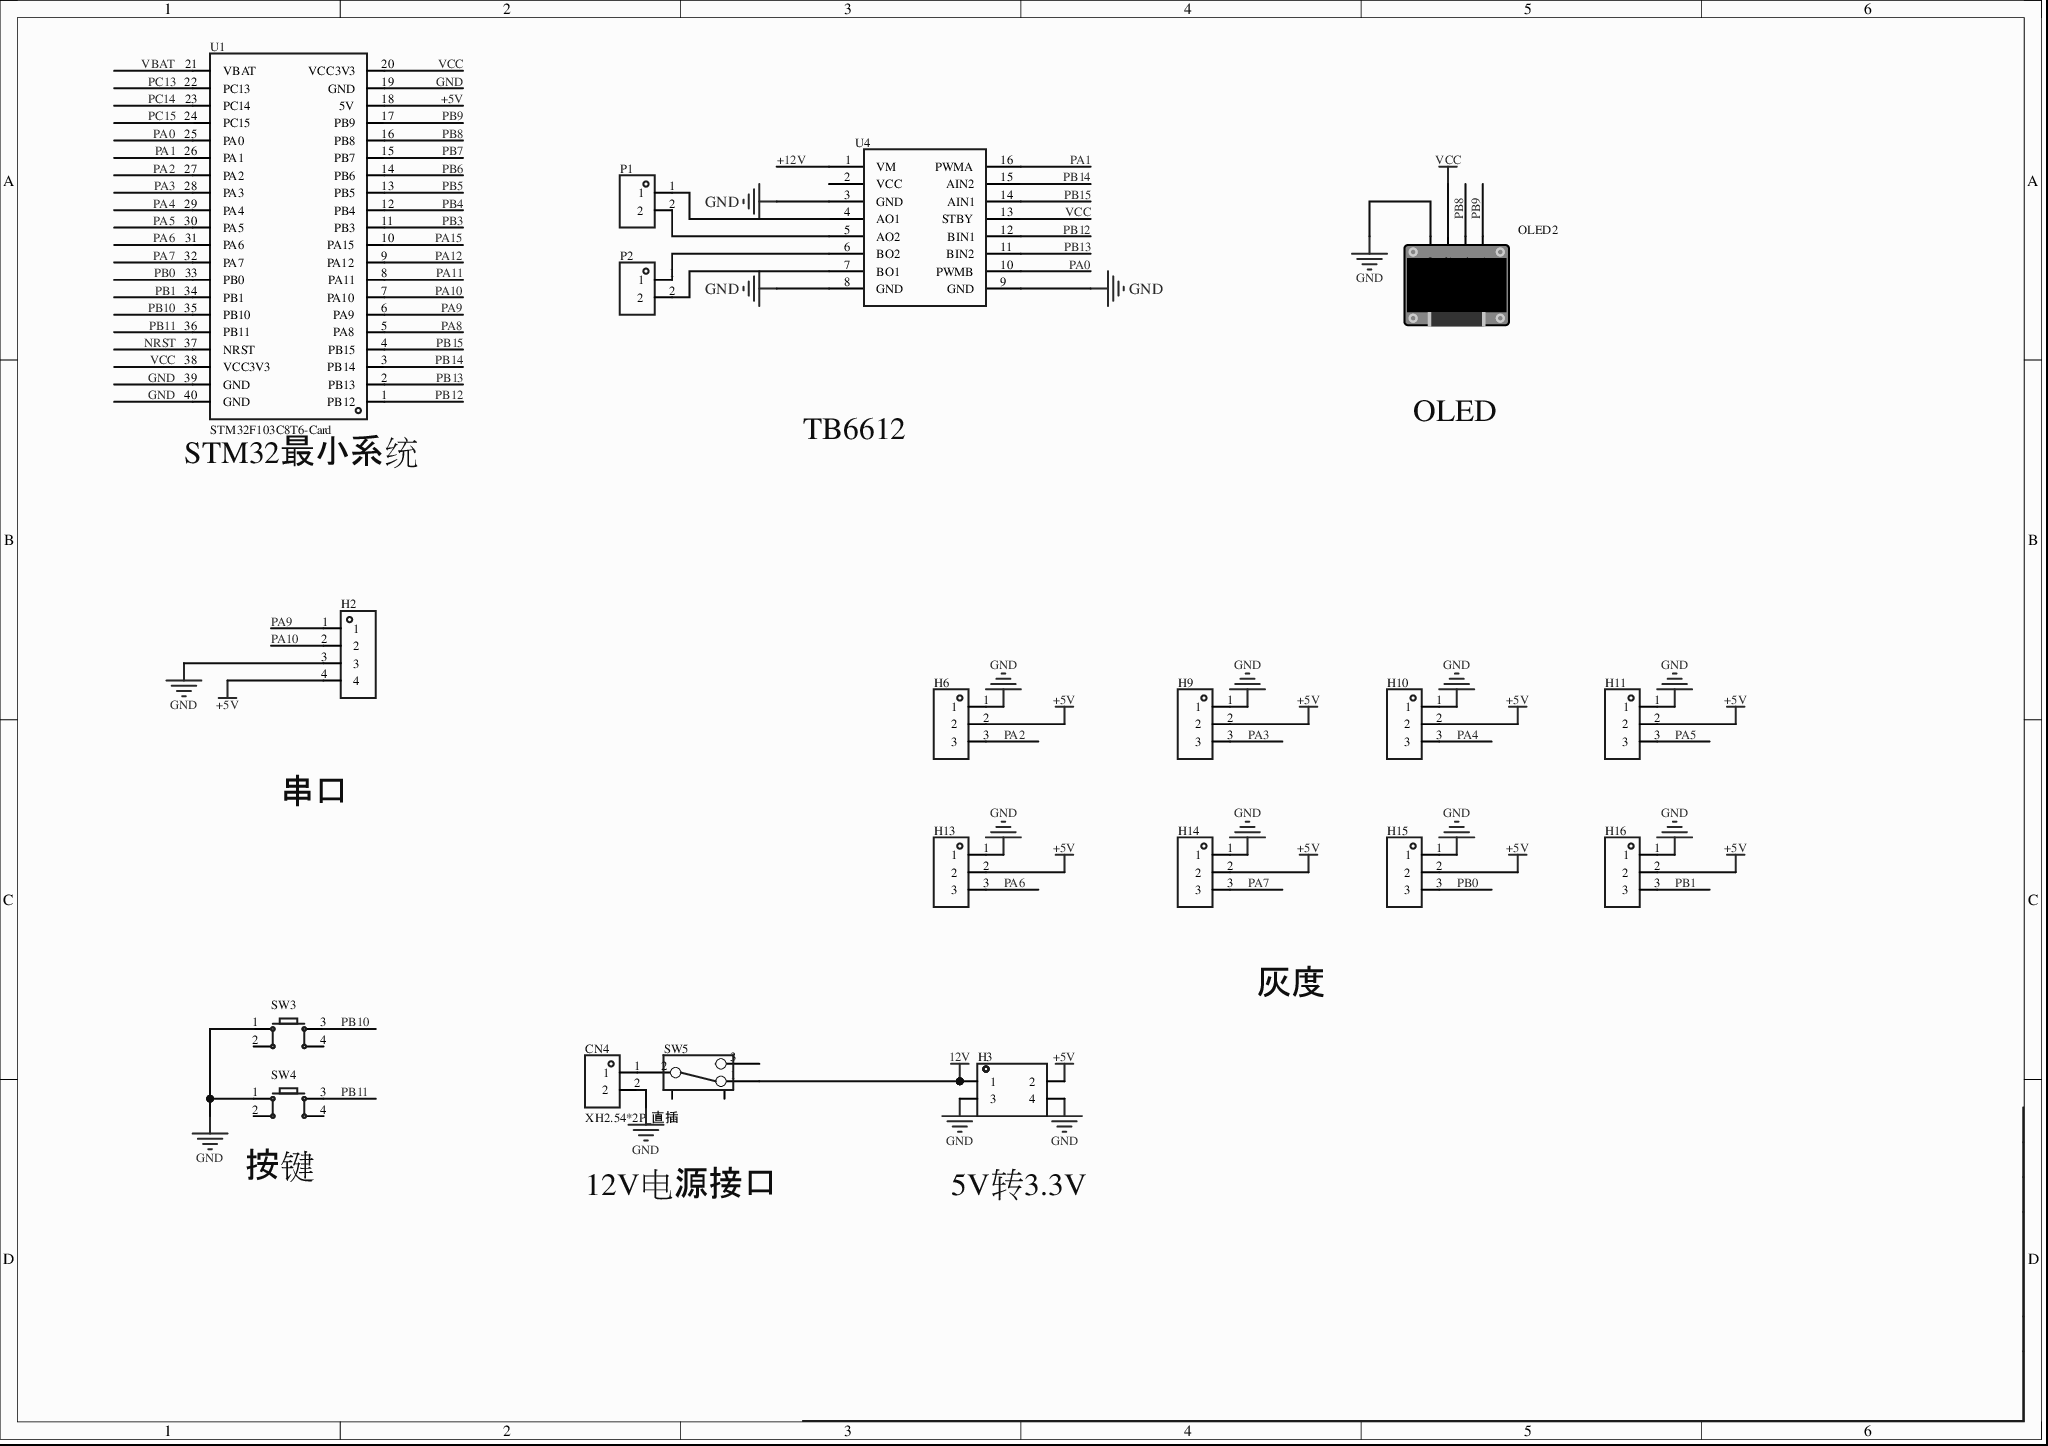
[diagram p0: MISC52001-3.schdoc]
# Altium project MISC52001-2.PrjPcb
1 sheet, 19 parts. Net scope: global (net labels, ports and power ports of the same name join across sheets).
Board file: MISC52001.pcbdoc

## Sheet MISC52001-3.schdoc
size 297 x 209 mm; Version: V1.0; @Project Name: MISC52001; @Page Count: 1; @Update Date: 2026-04-24; @Create Date: 2026-04-24; @Schematic Name: MISC52001; @Page No: 1; @Create Time: 23:22:16; @Update Time: 17:32:40; @Board Name: MISC52001

### Parts
CN4  XH2.54*2P_直插  [CONN-TH_2P-P2.50-XH2.54-2P]
H2  (no value)  [HDR-TH_4P-P2.54-V-M]
H3  (no value)  [HDR-TH_4P-P2.54-V-F-R2-C2-S2.54]
H6  (no value)  [HDR-TH_3P-P2.54-V-F]
H9  (no value)  [HDR-TH_3P-P2.54-V-F]
H10  (no value)  [HDR-TH_3P-P2.54-V-F]
H11  (no value)  [HDR-TH_3P-P2.54-V-F]
H13  (no value)  [HDR-TH_3P-P2.54-V-F]
H14  (no value)  [HDR-TH_3P-P2.54-V-F]
H15  (no value)  [HDR-TH_3P-P2.54-V-F]
H16  (no value)  [HDR-TH_3P-P2.54-V-F]
OLED2  (no value)  [0.96OLED_4P]
P1  KF301-2P接线端子  [CONN-TH_XY301V-A-5.0-2P]  (value not drawn)
P2  KF301-2P接线端子  [CONN-TH_XY301V-A-5.0-2P]  (value not drawn)
SW3  (no value)  [SW-TH_4P-L6.0-W6.0-P4.50-LS6.5]
SW4  (no value)  [SW-TH_4P-L6.0-W6.0-P4.50-LS6.5]
SW5  (no value)  [拨动开关]
U1  STM32F103C8T6-Card  [CONN-TH_L53.3-W22.9_STM32F103C8T6-CARD]
U4  (no value)  [tb6612]

### Nets
12V: H3.1 SW5.1
+5V: H2.4 H3.2 H6.2 H9.2 H10.2 H11.2 H13.2 H14.2 H15.2 H16.2 U1.18(5V)
GND: CN4.2 H2.3 H3.3 H3.4 H6.1 H9.1 H10.1 H11.1 H13.1 H14.1 H15.1 H16.1 OLED2.1(GND) SW3.1 SW4.1 U1.19(GND) U1.39(GND) U1.40(GND) U4.3(GND) U4.8(GND) U4.9(GND)
VCC: OLED2.2(VCC) U1.20(VCC3V3) U1.38(VCC3V3) U4.13(STBY)
+12V: U4.1(VM)
NRST: U1.37(NRST)
PA0: U1.25(PA0) U4.10(PWMB)
PA1: U1.26(PA1) U4.16(PWMA)
PA2: H6.3 U1.27(PA2)
PA3: H9.3 U1.28(PA3)
PA4: H10.3 U1.29(PA4)
PA5: H11.3 U1.30(PA5)
PA6: H13.3 U1.31(PA6)
PA7: H14.3 U1.32(PA7)
PA8: U1.5(PA8)
PA9: H2.1 U1.6(PA9)
PA10: H2.2 U1.7(PA10)
PA11: U1.8(PA11)
PA12: U1.9(PA12)
PA15: U1.10(PA15)
PB0: H15.3 U1.33(PB0)
PB1: H16.3 U1.34(PB1)
PB3: U1.11(PB3)
PB4: U1.12(PB4)
PB5: U1.13(PB5)
PB6: U1.14(PB6)
PB7: U1.15(PB7)
PB8: OLED2.3(SCL) U1.16(PB8)
PB9: OLED2.4(SDA) U1.17(PB9)
PB10: SW3.3 U1.35(PB10)
PB11: SW4.3 U1.36(PB11)
PB12: U1.1(PB12) U4.12(BIN1)
PB13: U1.2(PB13) U4.11(BIN2)
PB14: U1.3(PB14) U4.15(AIN2)
PB15: U1.4(PB15) U4.14(AIN1)
PC13: U1.22(PC13)
PC14: U1.23(PC14)
PC15: U1.24(PC15)
VBAT: U1.21(VBAT)
NetCN4_1: CN4.1 SW5.2
NetP1_1: P1.1 U4.4(AO1)
NetP1_2: P1.2 U4.5(AO2)
NetP2_1: P2.1 U4.6(BO2)
NetP2_2: P2.2 U4.7(BO1)

Not connected (* = marked no-connect by the designer): SW3 2 4; SW4 2 4; SW5 3 4 5; U4 2(VCC)

### Notes on the sheet
- DHT11温湿度模块：
  VCC   -》 3.3V
  DATA -》PB14
  GND  -》 GND
  hc06蓝牙模块：
  RXD -》 PA9
  TXD -》 PA10
  VCC -》 5V
  GND -》 GND
  土壤传感器模块：
  VCC  -》 3.3V
  GND -》 GND
  A0    -》 PA0
  蜂鸣器模块：
  IO 	-》PB5
  VCC  -》 5V
  GND -》GND
  OLED模块：
  SDA -> PB9
  SCL  -> PB8
  VCC -> 3.3v
  GND -> GND
  继电器模块：
  DC+ -》 5V
  DC-  -》 GND
  IN    -》 PB12
  按键模块：
  按键1 PC13
  按键2 PC14
  按键3 PC15
  按键4 PA1
  按键另外一端都接GND
  实物图：
  蜂鸣器：
- OLED
- (near U1) STM32最小系统
- TB6612
- 串口
- 灰度
- (near SW4) 按键
- 12V电源接口
- 5V转3.3V

### Library data of the parts
CN4 = XH2.54*2P_直插: 3D Model: 325c595e30db4df8abe76612dd40b0fa0819f05c4eef4c71ace90d822a990e87; 3D Model Transform: 295.275,228.346,0,180,0,0,-0.002,-20.079,-137.795; AddInBom: yes; Device: XH2.54*2P_直插; Symbol: XH2.54*2P_直插; LCSC Part Name: XH2.54*2P_直插; Supplier Part: C9900008615; Manufacturer Part: XH2.54*2P_直插; Supplier Footprint: XH2.54_2P; JLCPCB Part Class: Extended Part; Supplier: LCSC; FootprintName: CONN-TH_2P-P2.50-XH2.54-2P; ConvertToPcb: yes; ModelName: CONN-TH_2P-P2.50-XH2.54-2P
H2 = HDR-M_2.54_1x4P: Symbol: PZ254V-11-04P; ConvertToPcb: yes; ModelId: 112f4d05e8d64e99ab9a333894bea4f90819f05c4eef4c71ace90d822a990e87; ModelName: HDR-TH_4P-P2.54-M-LI-1X4P; ModelTransform: 399.999,104.7242,0,0,0,0,0,0,-118.11; Device: HDR-M_2.54_1x4P; AddInBom: yes; SupplierPart: C492403; Supplier Footprint: 插件; FootprintName: HDR-TH_4P-P2.54-V-M
H3 = HDR-F_2.54_2x2: Symbol: HDR-F-2.54_2x2; 3D Model: 870c884146ee4765973edc845f10b7af0819f05c4eef4c71ace90d822a990e87; 3D Model Transform: 215.7476,196.85,0,0,0,0,0,0,-118.11; ConvertToPcb: yes; ModelName: HDR-TH_4P-P2.54-F-LI-2X2P; Device: HDR-F_2.54_2x2; Supplier Part: C92273; Supplier Footprint: 插件; AddInBom: yes; FootprintName: HDR-TH_4P-P2.54-V-F-R2-C2-S2.54
H6 H9-H11 H13-H16 = HDR-F_2.54_1x3P: Symbol: PM254V-11-03-H85; 3D Model: f3b3cc5aae9641bf9e56fc160cef875b; 3D Model Transform: 299.9994,100,0,0,0,0,0,0,-118.11; ConvertToPcb: yes; ModelName: HDR2.54-F-LI-1X3P; Device: HDR-F_2.54_1x3P; Supplier Part: C541850; Supplier Footprint: 插件; FootprintName: HDR-TH_3P-P2.54-V-F; AddInBom: yes
OLED2 = 0.96OLED模块_4P: ConvertToPcb: yes; ModelId: 79c000fdb68d45a296c2e9bedf4f9055; ModelTransform: 1393.69792,1318.895,0,0,0,0,0,-560.079,-137.795; Symbol: 0.96OLED模块_4P; Device: 0.96OLED模块_4P; AddInBom: yes; FootprintName: 0.96OLED_4P; Supplier Footprint: 插件; ModelName: 0.96OLED_4P
P1 P2 = KF301-2P接线端子: 3D Model: ef7ead88b0f2448d904975b26718870f; 3D Model Transform: 417.322,299.212,0,0,0,0,11.811,-7.835,-157.48; AddInBom: yes; Symbol: KF301-2P接线端子; Device: KF301-2P接线端子; LCSC Part Name: KF301-2P接线端子; Supplier Part: C9900016950; Manufacturer Part: KF301-2P接线端子; Supplier Footprint: CK301-2P; Supplier: LCSC; ConvertToPcb: yes; FootprintName: CONN-TH_XY301V-A-5.0-2P; ModelName: CONN-TH_XY301V-A-5.0-2P
SW3 SW4 = Key_TH_6x6x6: 触点电流:50mA;额定电压(DC):12V;绝缘电阻:100MΩ;电路结构:单刀单掷;安装方式:直插;按钮形状:圆形按钮;按钮/盖帽颜色:黑色;作用力:260gf@±30gf;工作温度:-25℃~+70℃;引脚样式:PC引脚;开关长度:6mm;开关宽度:6mm;开关高度:6mm;带支架:否;; Symbol: 轻触按键; AddInBom: yes; ModelId: 20eee248bc684ccd8cbdbb1d0d91ec6f0819f05c4eef4c71ace90d822a990e87; ModelName: SW-TH_4P-L6.0-W6.0-H5.0-LS6.5-P4.50; ModelTransform: 236.22,323.03,0,90,0,0,0,0,-137.795; Device: Key_TH_6x6x6; FootprintName: SW-TH_4P-L6.0-W6.0-P4.50-LS6.5; ConvertToPcb: yes; Supplier Footprint: 插件
SW5 = 拨动开关_正: ConvertToPcb: yes; ModelId: 4321fe59a4074cbfb4989553f297c68f0819f05c4eef4c71ace90d822a990e87; ModelName: SW-TH_SS-12D02-VG4; ModelTransform: 370.09,208.7,472.35,0,0,0,0,0,-110; Device: 拨动开关_正; Symbol: 拨动开关; FootprintName: 拨动开关; AddInBom: yes; Supplier Footprint: 插件
U1 = STM32F103C8T6-Card: AddInBom: yes; Device: STM32F103C8T6-Card; Symbol: STM32F103C8T6-CARD; FootprintName: CONN-TH_L53.3-W22.9_STM32F103C8T6-CARD; LCSC Part Name: STM32F103C8T6-Card; SupplierPart: C9900077949; ManufacturerPart: STM32F103C8T6-Card; Supplier Footprint: 插件; Supplier: LCSC; ConvertToPcb: yes
U4 = tb6612: AddInBom: yes; Symbol: tb6612; Device: tb6612; JLCPCB Part Class: 扩展库; ConvertToPcb: yes; FootprintName: tb6612